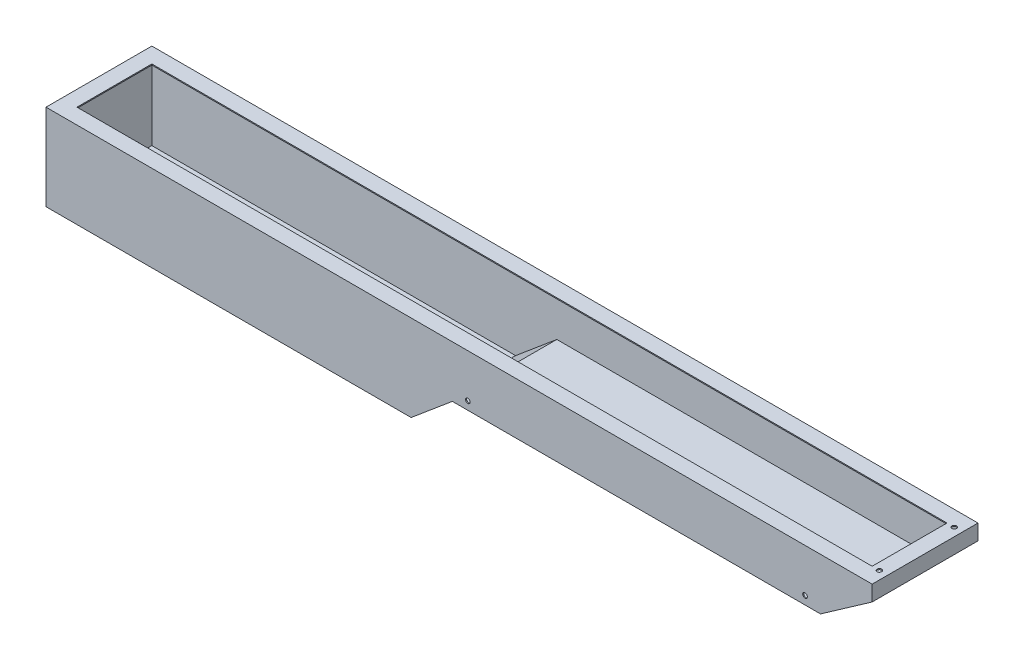
from build123d import *

# Parameters (mm, degrees)
EXTRUDE_1_DEPTH     = 205
SHELL_1_T           = -2
SKETCH_4_W          = 1600
SKETCH_4_H          = 205
SKETCH_4_W_2        = 1540
SKETCH_4_H_2        = 145
EXTRUDE_2_DEPTH     = 2
SKETCH_5_R          = 4.5
CUT_EXTRUDE_1_DEPTH = 2
SKETCH_7_R          = 4.5
CUT_EXTRUDE_2_DEPTH = 78
SKETCH_8_R          = 4.5
CUT_EXTRUDE_3_DEPTH = 16
SKETCH_9_R          = 4.5
CUT_EXTRUDE_4_DEPTH = 110


with BuildPart() as part:
    # 草图2 → 凸台-拉伸1 (new body)
    with BuildSketch(Plane(origin=(0, 0, 0), x_dir=(-1, 0, 0), z_dir=(0, 0, -1))):
        Polygon((-1600, -30), (-1500.029639528, -100), (-787, -100), (-707.152509296, -167), (0, -167), (0, 0), (-1600, 0), align=None)
    extrude(amount=EXTRUDE_1_DEPTH)

    # 抽壳1
    shell_1_openings = [part.faces().sort_by_distance(p)[0] for p in [
        (800, 0, -102.5),
    ]]
    offset(amount=SHELL_1_T, openings=shell_1_openings, kind=Kind.INTERSECTION)

    # 草图4 → 凸台-拉伸2 (add)
    with BuildSketch(Plane(origin=(0, 0, 0), x_dir=(1, 0, 0), z_dir=(0, 1, 0))):
        with Locations((800, 102.5)):
            Rectangle(SKETCH_4_W, SKETCH_4_H)
        with Locations((800, 102.5)):
            Rectangle(SKETCH_4_W_2, SKETCH_4_H_2, mode=Mode.SUBTRACT)
    extrude(amount=-EXTRUDE_2_DEPTH)

    # 草图5 → 切除-拉伸1 (cut)
    with BuildSketch(Plane(origin=(0, 0, -205), x_dir=(-1, 0, 0), z_dir=(0, 0, -1))):
        with Locations((-1570, -14)):
            Circle(SKETCH_5_R)
        with Locations((-30, -14)):
            Circle(SKETCH_5_R)
        with Locations((-800, -14)):
            Circle(SKETCH_5_R)
    extrude(amount=-CUT_EXTRUDE_1_DEPTH, mode=Mode.SUBTRACT)

    # 草图7 → 切除-拉伸2 (cut)
    with BuildSketch(Plane.ZY):
        with Locations((-175, -151)):
            Circle(SKETCH_7_R)
        with Locations((-30, -151)):
            Circle(SKETCH_7_R)
    extrude(amount=-CUT_EXTRUDE_2_DEPTH, mode=Mode.SUBTRACT)

    # 草图8 → 切除-拉伸3 (cut)
    with BuildSketch(Plane(origin=(0, 0, 0), x_dir=(1, 0, 0), z_dir=(0, 1, 0))):
        with Locations(Location((1584, 175, 0), (0, 0, 180))):
            Circle(SKETCH_8_R)
        with Locations(Location((1584, 30, 0), (0, 0, 180))):
            Circle(SKETCH_8_R)
    extrude(amount=-CUT_EXTRUDE_3_DEPTH, mode=Mode.SUBTRACT)

    # 草图9 → 切除-拉伸4 (cut)
    with BuildSketch(Plane.XY):
        with Locations((817, -84)):
            Circle(SKETCH_9_R)
        with Locations((1470.029639528, -84)):
            Circle(SKETCH_9_R)
    extrude(amount=-CUT_EXTRUDE_4_DEPTH, mode=Mode.SUBTRACT)


solid = part.part
